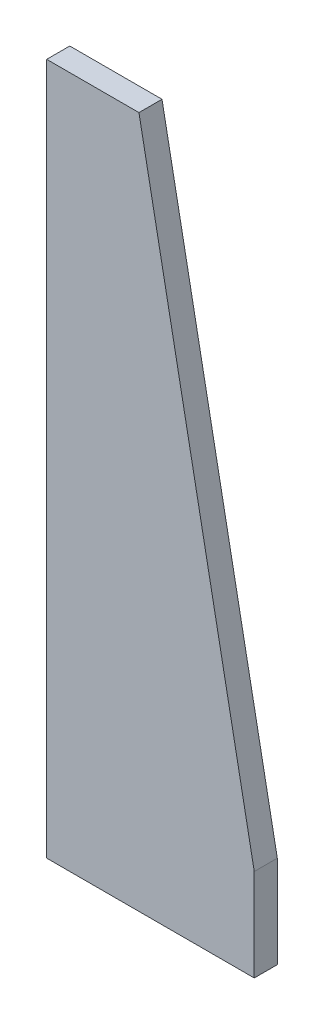
SolidWorks part; units mm, degrees
material "5.0热板"
ref_plane "前视" through (0, 0, 0) normal (0, 0, 1) x (1, 0, 0)
ref_plane "上视" through (0, 0, 0) normal (0, 1, 0) x (1, 0, 0)
ref_plane "右视" through (0, 0, 0) normal (1, 0, 0) x (0, 0, -1)
sketch "草图1" plane through (0, 0, 0) normal (0, 0, 1) x (1, 0, 0)
  line L0 (0, 0) -> (0, 150)
  line L1 (0, 150) -> (20, 150)
  line L2 (20, 150) -> (45, 20)
  line L3 (45, 20) -> (45, 0)
  line L4 (45, 0) -> (0, 0)
  dimension "D1" = 45
  dimension "D2" = 20
  dimension "D3" = 150
  dimension "D4" = 20
extrude "凸台-拉伸1" add sketch "草图1" along normal mid plane 5
